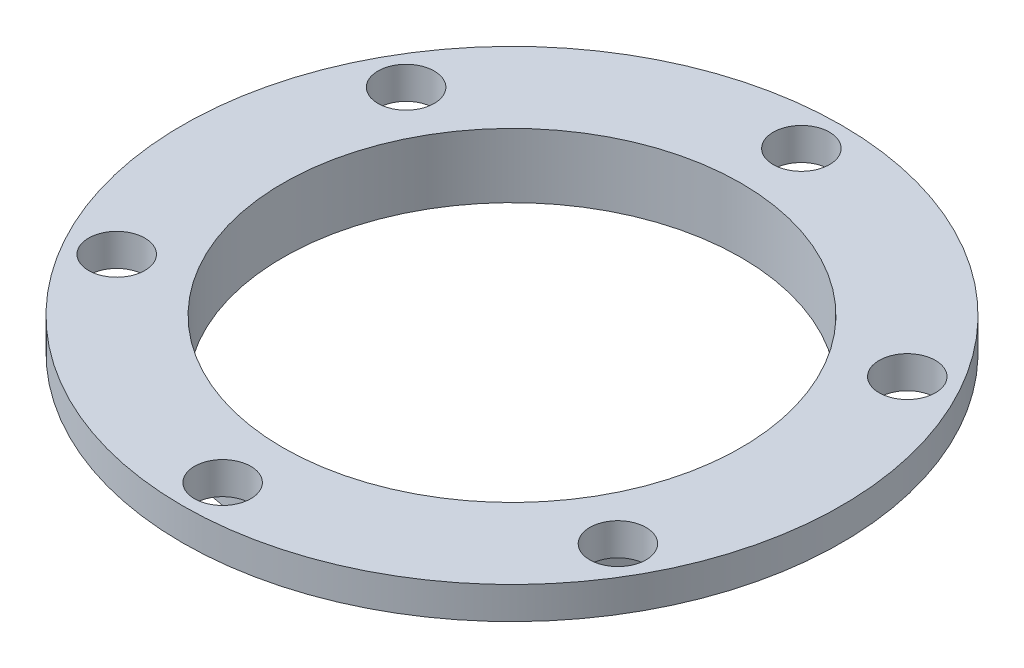
SolidWorks part; units mm, degrees
material "普通碳钢"
ref_plane "Front Plane" through (0, 0, 0) normal (0, 0, 1) x (1, 0, 0)
ref_plane "Top Plane" through (0, 0, 0) normal (0, 1, 0) x (1, 0, 0)
ref_plane "Right Plane" through (0, 0, 0) normal (1, 0, 0) x (0, 0, -1)
ref_plane "Plane1" through (0, 0, 89.5) normal (0, 0, 1) x (1, 0, 0)
sketch "Sketch1" plane through (0, 0, 89.5) normal (0, 0, 1) x (1, 0, 0)
  line L0 (-1028.592, 74.4724) -> (-1069.592, 74.4724)
  line L1 (-1069.592, 74.4724) -> (-1069.592, 70.4724)
  line L2 (-1069.592, 70.4724) -> (-1028.592, 70.4724)
  line L3 (-1028.592, 70.4724) -> (-1028.592, 74.4724)
  line L4 (-1069.592, 74.4724) -> (-1069.592, 70.4724) construction
  dimension "D1" = 41
revolve "Revolve1" add sketch "Sketch1" angle 360 about L4
sketch "Sketch2" plane through (0, 70.4724, 0) normal (0, -1, 0) x (1, 0, 0)
  circle A0 centre (-1069.592, 89.5) radius 31
extrude "Boss-Extrude1" add sketch "Sketch2" along normal blind 4
hole_wizard "M52 Clearance Hole1" positions "Sketch4" profile "Sketch3" hole size "M52" standard "ANSI Metric"
sketch "Sketch4" plane through (0, 66.4724, 0) normal (0, -1, 0) x (-1, 0, 0)
  point P0 (1069.592, -89.5)
sketch "Sketch3" plane through (-1069.592, 66.4724, 89.5) normal (1, 0, 0) x (0, 0, -1)
  line L0 (0, 0) -> (0, 8)
  line L1 (0, 8) -> (28.5, 8)
  line L2 (28.5, 8) -> (28.5, 0)
  line L5 (28.5, 0) -> (0, 0)
  line L11 (0, -6.35) -> (0, 107.95) construction
  dimension "通孔孔直径" = 57
  dimension "通孔孔深度" = 8
hole_wizard "Ø7.0 (7) Diameter Hole1" positions "Sketch6" profile "Sketch5" hole size "Ø7.0" standard "ANSI Metric"
sketch "Sketch6" plane through (0, 70.4724, 0) normal (0, -1, 0) x (-1, 0, 0)
  line L0 (1038.4151, -71.5) -> (1102.501, -108.5) construction
  line L2 (1100.7689, -71.5) -> (1038.4151, -107.5) construction
  line L4 (1069.592, -53.5) -> (1069.592, -125.5) construction
  circle A0 centre (1069.592, -89.5) radius 36 construction
  point P0 (1069.592, -125.5)
  point P1 (1100.7689, -107.5)
  point P2 (1100.7689, -71.5)
  point P3 (1069.592, -53.5)
  point P4 (1038.4151, -71.5)
  point P5 (1038.4151, -107.5)
  dimension "D1" = 72
  dimension "D2" = 60
  dimension "D3" = 60
sketch "Sketch5" plane through (-1069.592, 70.4724, 125.5) normal (1, 0, 0) x (0, 0, -1)
  line L0 (0, 0) -> (0, 4)
  line L1 (0, 4) -> (3.5, 4)
  line L2 (3.5, 4) -> (3.5, 0)
  line L5 (3.5, 0) -> (0, 0)
  line L11 (0, -6.35) -> (0, 107.95) construction
  dimension "通孔孔直径" = 7
  dimension "通孔孔深度" = 4
ref_plane "Plane2" through (-1110.592, 0, 0) normal (-1, 0, 0) x (0, 0, 1)
ref_plane "Plane3" through (-1028.592, 0, 0) normal (1, 0, 0) x (0, 0, -1)
ref_plane "Plane4" through (-1069.592, 0, 0) normal (-1, 0, 0) x (0, 0, 1)
